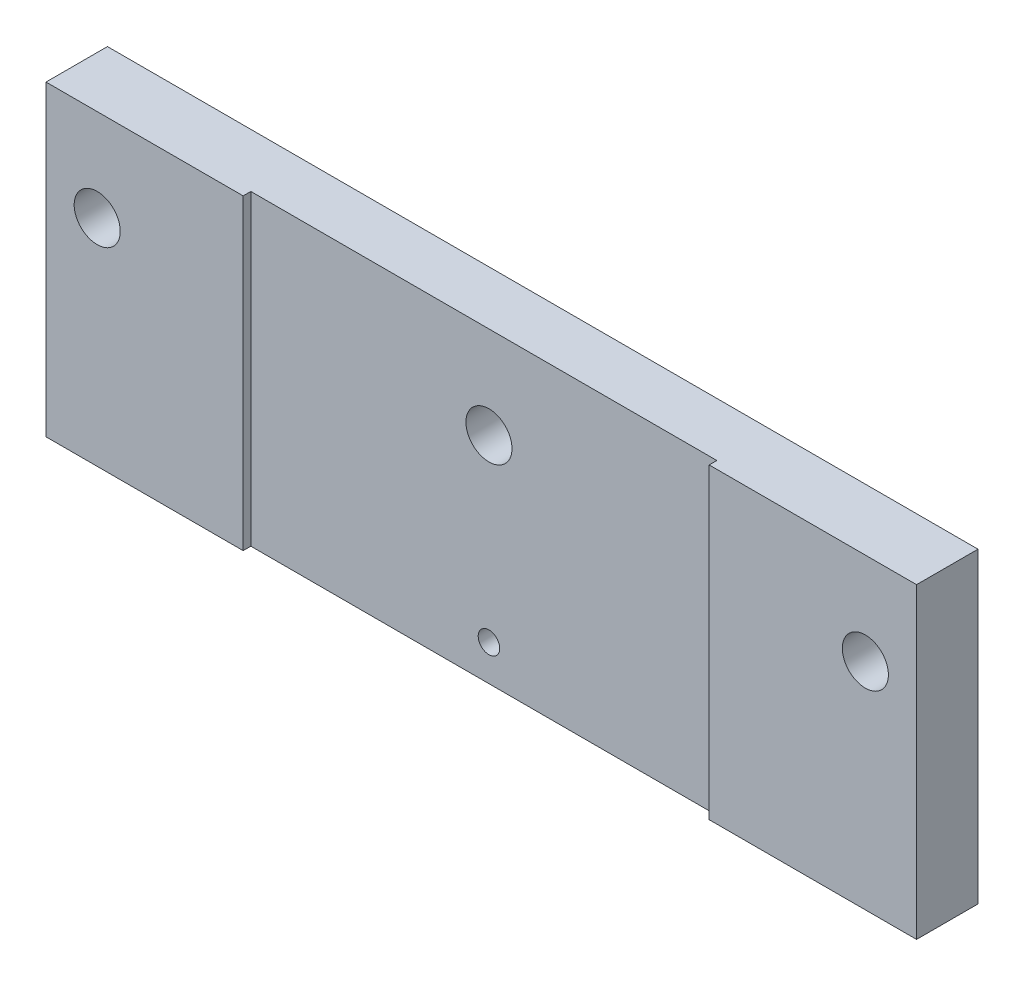
from build123d import *

# Parameters (mm, degrees)
SKETCH_1_W                   = 170
SKETCH_1_H                   = 60
SKETCH_1_R                   = 4.5
EXTRUDE_1_DEPTH              = 6
SKETCH_2_W                   = 91
SKETCH_2_H                   = 60
CUT_EXTRUDE_1_DEPTH          = 1.5
HOLE_WIZARD_M5_1_D           = 4.2
HOLE_WIZARD_M5_1_CSINK_D     = 5.05
HOLE_WIZARD_M5_1_CSINK_ANGLE = 90


with BuildPart() as part:
    # 草图1 → 凸台-拉伸1 (new, symmetric)
    with BuildSketch(Plane.XY):
        Rectangle(SKETCH_1_W, SKETCH_1_H)
        with Locations((-75, 12)):
            Circle(SKETCH_1_R, mode=Mode.SUBTRACT)
        with Locations((75, 12)):
            Circle(SKETCH_1_R, mode=Mode.SUBTRACT)
        with Locations((0, 12)):
            Circle(SKETCH_1_R, mode=Mode.SUBTRACT)
    extrude(amount=EXTRUDE_1_DEPTH, both=True)

    # 草图2 → 切除-拉伸1 (cut)
    with BuildSketch(Plane.XY.offset(6)):
        with Locations((-1, 0)):
            Rectangle(SKETCH_2_W, SKETCH_2_H)
    extrude(amount=-CUT_EXTRUDE_1_DEPTH, mode=Mode.SUBTRACT)

    # M5 螺纹孔1 (through all)
    with Locations(Plane(origin=(0, -23, -6), x_dir=(-1, 0, 0), z_dir=(0, 0, -1))):
        with Locations((0, 0)):
            CounterSinkHole(HOLE_WIZARD_M5_1_D / 2, HOLE_WIZARD_M5_1_CSINK_D / 2, counter_sink_angle=HOLE_WIZARD_M5_1_CSINK_ANGLE)


solid = part.part
